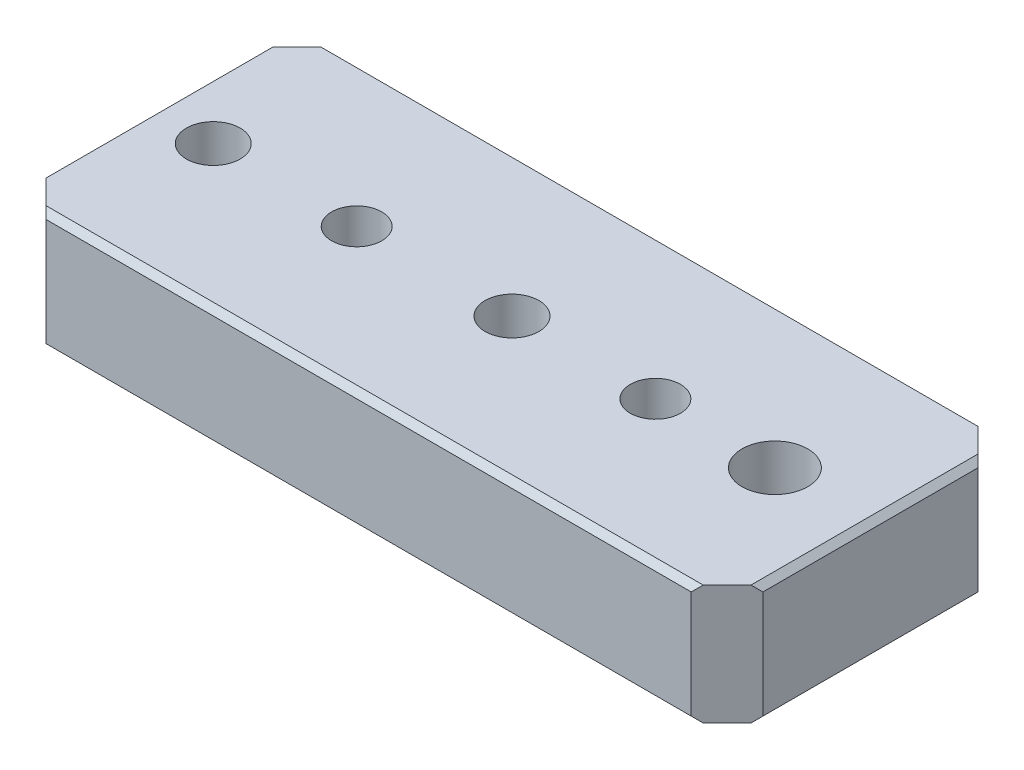
SolidWorks part; units mm, degrees
material "A6061"
ref_plane "Front Plane" through (0, 0, 0) normal (0, 0, 1) x (1, 0, 0)
ref_plane "Top Plane" through (0, 0, 0) normal (0, 1, 0) x (1, 0, 0)
ref_plane "Right Plane" through (0, 0, 0) normal (1, 0, 0) x (0, 0, -1)
sketch "Sketch1" plane through (0, 0, 0) normal (0, 1, 0) x (1, 0, 0)
  line L1 (-28.9271, 8.8363) -> (26.0729, 8.8363)
  line L2 (-28.9271, 8.8363) -> (-28.9271, -15.1637)
  line L3 (-28.9271, -15.1637) -> (26.0729, -15.1637)
  line L4 (26.0729, 8.8363) -> (26.0729, -15.1637)
  dimension "D1" = 55
  dimension "D2" = 24
  dimension "D3" = 15.1637
  dimension "D4" = 26.0729
extrude "Boss-Extrude1" add sketch "Sketch1" along normal blind 10
hole_wizard "Hole Size (Based On) Socket Head Cap Screw Type3" positions "Sketch3" profile "Sketch2" counterbore size "M5" standard "GB"
sketch "Sketch3" plane through (0, 0, 0) normal (0, -1, 0) x (-1, 0, 0)
  line L7 (-26.0729, 9.8363) -> (38.9271, 9.8363) construction
  line L8 (-26.0729, -15.1637) -> (-26.0729, 9.8363) construction
  point P4 (-19.0729, -1.1637)
  point P25 (-26.0729, -2.6637)
  dimension "D1" = 11
  dimension "D2" = 7
sketch "Sketch2" plane through (19.0729, 0, 1.1637) normal (1, 0, 0) x (0, 0, -1)
  line L0 (0, 0) -> (0, 14.0524)
  line L1 (0, 14.0524) -> (2.75, 12.4)
  line L2 (2.75, 12.4) -> (2.75, 5.7)
  line L3 (2.75, 5.7) -> (5, 5.7)
  line L4 (5, 5.7) -> (5, 0)
  line L5 (5, 0) -> (0, 0)
  line L10 (0, 14.0524) -> (-2.75, 12.4) construction
  line L11 (0, -6.35) -> (0, 107.95) construction
  dimension "孔直径" = 5.5
  dimension "孔深度" = 12.4
  dimension "柱形沉头孔直径" = 10
  dimension "柱形沉头孔深度" = 5.7
  dimension "导头角度" = 118
hole_wizard "打孔尺寸(%根据)内六角圆柱头螺钉的类型3" positions "Sketch5" profile "Sketch4" counterbore size "M4" standard "GB"
sketch "Sketch5" plane through (0, 0, 0) normal (0, -1, 0) x (-1, 0, 0)
  line L4 (-1.0729, -3.1637) -> (23.9271, -3.1637)
  line L8 (-26.0729, -15.1637) -> (-26.0729, 8.8363) construction
  line L9 (28.9271, -15.1637) -> (-26.0729, -15.1637) construction
  point P0 (23.9271, -3.1637)
  point P3 (-1.0729, -3.1637)
  dimension "D1" = 25
  dimension "D2" = 25
  dimension "D3" = 12
sketch "Sketch4" plane through (-23.9271, 0, 3.1637) normal (1, 0, 0) x (0, 0, -1)
  line L0 (0, 0) -> (0, 13.7519)
  line L1 (0, 13.7519) -> (2.25, 12.4)
  line L2 (2.25, 12.4) -> (2.25, 4.6)
  line L3 (2.25, 4.6) -> (4, 4.6)
  line L4 (4, 4.6) -> (4, 0)
  line L5 (4, 0) -> (0, 0)
  line L10 (0, 13.7519) -> (-2.25, 12.4) construction
  line L11 (0, -6.35) -> (0, 107.95) construction
  dimension "孔直径" = 4.5
  dimension "孔深度" = 12.4
  dimension "柱形沉头孔直径" = 8
  dimension "柱形沉头孔深度" = 4.6
  dimension "导头角度" = 118
sketch "Sketch6" plane through (0, 0, 0) normal (0, -1, 0) x (1, 0, 0)
  line L1 (26.0729, 15.1637) -> (31.0729, 15.1637)
  line L2 (26.0729, 15.1637) -> (26.0729, -8.8363)
  line L3 (26.0729, -8.8363) -> (31.0729, -8.8363)
  line L4 (31.0729, 15.1637) -> (31.0729, -8.8363)
  line M7 (26.0729, -8.8363) -> (26.0729, 15.1637)
  dimension "D1" = 5
extrude "Boss-Extrude2" add sketch "Sketch6" against normal up to surface (10 mm away) contours L4 L1 L3 M7 up to face at (-23.9271, 10, 5.4137)
chamfer "Chamfer1" distance 3 angle 45 4 edges at (31.0729, 5, -8.8363) (31.0729, 5, 15.1637) (-28.9271, 5, 15.1637) (-28.9271, 5, -8.8363)
chamfer "Chamfer2" distance 0.5 angle 45 8 edges at (31.0729, 0, 3.1637) (31.0729, 10, 3.1637) (1.0729, 0, 15.1637) (1.0729, 10, 15.1637) (-28.9271, 0, 3.1637) (-28.9271, 10, 3.1637) (1.0729, 0, -8.8363) (1.0729, 10, -8.8363)
hole_wizard "Hole Size (Based On) Socket Head Cap Screw Type4" positions "Sketch12" profile "Sketch11" counterbore size "M5" standard "GB"
sketch "Sketch12" plane through (0, 0, 0) normal (0, -1, 0) x (-1, 0, 0)
  line L0 (-31.0729, -12.1637) -> (-31.0729, 5.8363) construction
  line L1 (-28.0729, 8.8363) -> (25.9271, 8.8363) construction
  point P0 (-23.0729, -3.1637)
  dimension "D1" = 8
  dimension "D2" = 12
sketch "Sketch11" plane through (23.0729, 0, 3.1637) normal (1, 0, 0) x (0, 0, -1)
  line L0 (0, 0) -> (0, 14.0524)
  line L1 (0, 14.0524) -> (2.75, 12.4)
  line L2 (2.75, 12.4) -> (2.75, 5.7)
  line L3 (2.75, 5.7) -> (5, 5.7)
  line L4 (5, 5.7) -> (5, 0)
  line L5 (5, 0) -> (0, 0)
  line L10 (0, 14.0524) -> (-2.75, 12.4) construction
  line L11 (0, -6.35) -> (0, 107.95) construction
  dimension "孔直径" = 5.5
  dimension "孔深度" = 12.4
  dimension "柱形沉头孔直径" = 10
  dimension "柱形沉头孔深度" = 5.7
  dimension "导头角度" = 118
hole_wizard "M5 Tapped Hole1" positions "Sketch10" profile "Sketch9" tap size "M5" standard "GB" end condition through all
sketch "Sketch10" plane through (0, 10, 0) normal (0, 1, 0) x (1, 0, 0)
  line L0 (-11.9271, -3.1637) -> (13.0729, -3.1637)
  line L4 (31.0729, 5.8363) -> (31.0729, -12.1637) construction
  line L5 (28.0729, -15.1637) -> (-25.9271, -15.1637) construction
  point P0 (-11.9271, -3.1637)
  point P2 (13.0729, -3.1637)
  dimension "D1" = 18
  dimension "D2" = 25
  dimension "D3" = 12
sketch "Sketch9" plane through (-11.9271, 10, 3.1637) normal (1, 0, 0) x (0, 0, 1)
  line L0 (0, 0) -> (0, 10)
  line L1 (0, 10) -> (2.1, 10)
  line L2 (2.1, 10) -> (2.1, 0)
  line L5 (2.1, 0) -> (0, 0)
  line L11 (0, -6.35) -> (0, 107.95) construction
  dimension "通孔螺纹孔钻头直径" = 4.2
  dimension "通孔螺纹孔钻头深度" = 10
cosmetic thread "Cosmetic Thread1" parameters "D2"=5
cosmetic thread "Cosmetic Thread2" parameters "D2"=5
